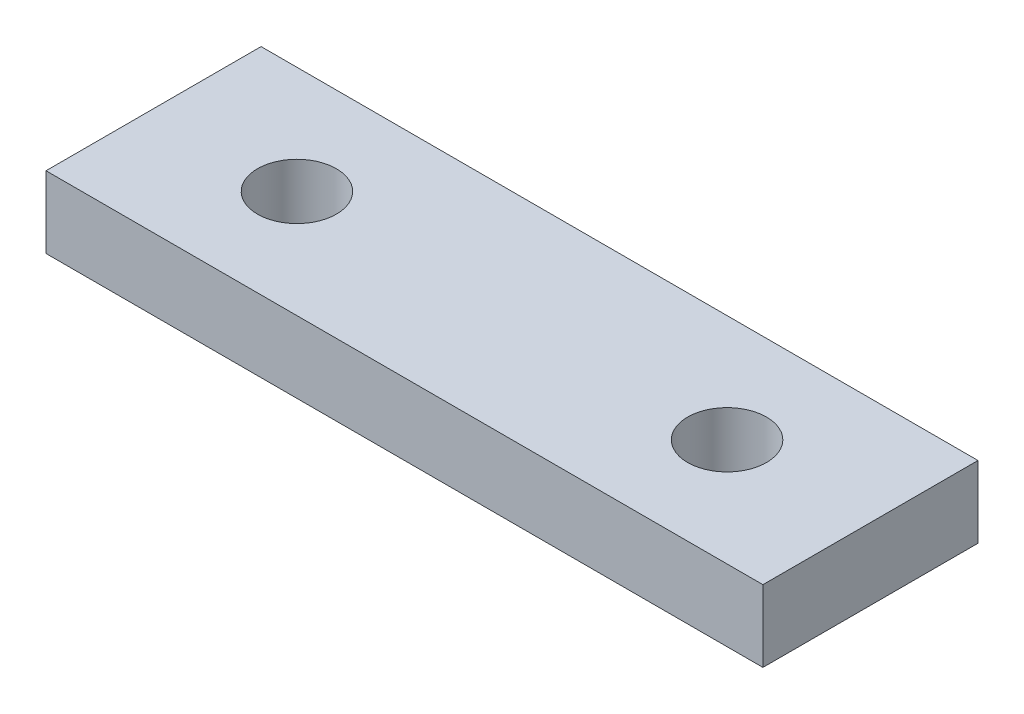
from build123d import *

# Parameters (mm, degrees)
SKETCH1_W                  = 100
SKETCH1_H                  = 30
BOSS_EXTRUDE1_DEPTH        = 10
F_11_0_11_DIAMETER_HOLE1_D = 11


with BuildPart() as part:
    # Sketch1 → Boss-Extrude1 (new body)
    with BuildSketch(Plane(origin=(0, 0, 0), x_dir=(1, 0, 0), z_dir=(0, 1, 0))):
        Rectangle(SKETCH1_W, SKETCH1_H)
    extrude(amount=BOSS_EXTRUDE1_DEPTH)

    # Ø11.0 (11) Diameter Hole1 (through all)
    with Locations(Plane(origin=(0, 10, 0), x_dir=(1, 0, 0), z_dir=(0, 1, 0))):
        with Locations((-30, 0), (30, 0)):
            Hole(F_11_0_11_DIAMETER_HOLE1_D / 2)


solid = part.part
